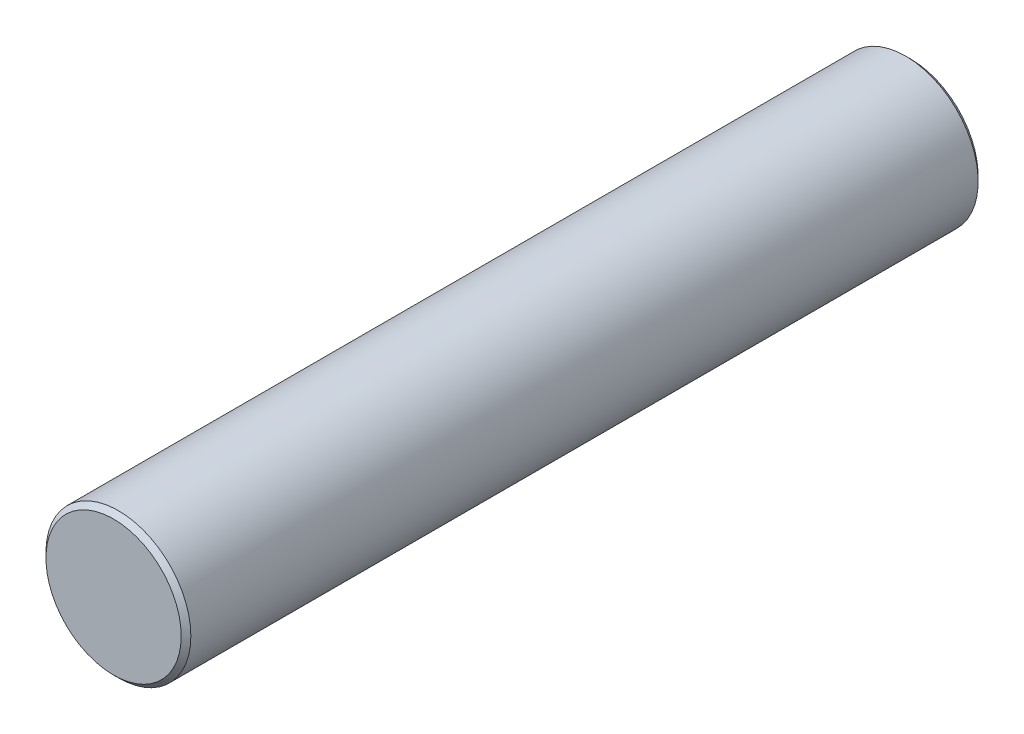
SolidWorks part; units mm, degrees
ref_plane "Front Plane" through (0, 0, 0) normal (0, 0, 1) x (1, 0, 0)
ref_plane "Top Plane" through (0, 0, 0) normal (0, 1, 0) x (1, 0, 0)
ref_plane "Right Plane" through (0, 0, 0) normal (1, 0, 0) x (0, 0, -1)
sketch "Sketch1" plane through (0, 0, 0) normal (0, 0, 1) x (1, 0, 0)
  circle A0 centre (0, 0) radius 3
  dimension "D1" = 6
extrude "Boss-Extrude1" add sketch "Sketch1" along normal mid plane 33
chamfer "Chamfer1" distance 0.2 angle 45 2 edges at (3, 0, -16.5) (3, 0, 16.5)
sketch "Sketch2" plane through (0, 0, 0) normal (0, 1, 0) x (1, 0, 0)
  line L0 (-3, 16.3) -> (-3, -16.3) construction
  line L1 (-3, 16.5) -> (-2.5, 16.5)
  line L2 (-3, 16.5) -> (-3, 6.5)
  line L3 (-3, 6.5) -> (-2.5, 6.5)
  line L4 (-2.5, 16.5) -> (-2.5, 6.5)
  line L5 (2.8, 16.5) -> (-2.8, 16.5) construction
  dimension "D1" = 10
  dimension "D2" = 0.5
extrude "Cut-Extrude1" cut sketch "Sketch2" against normal mid plane 30
